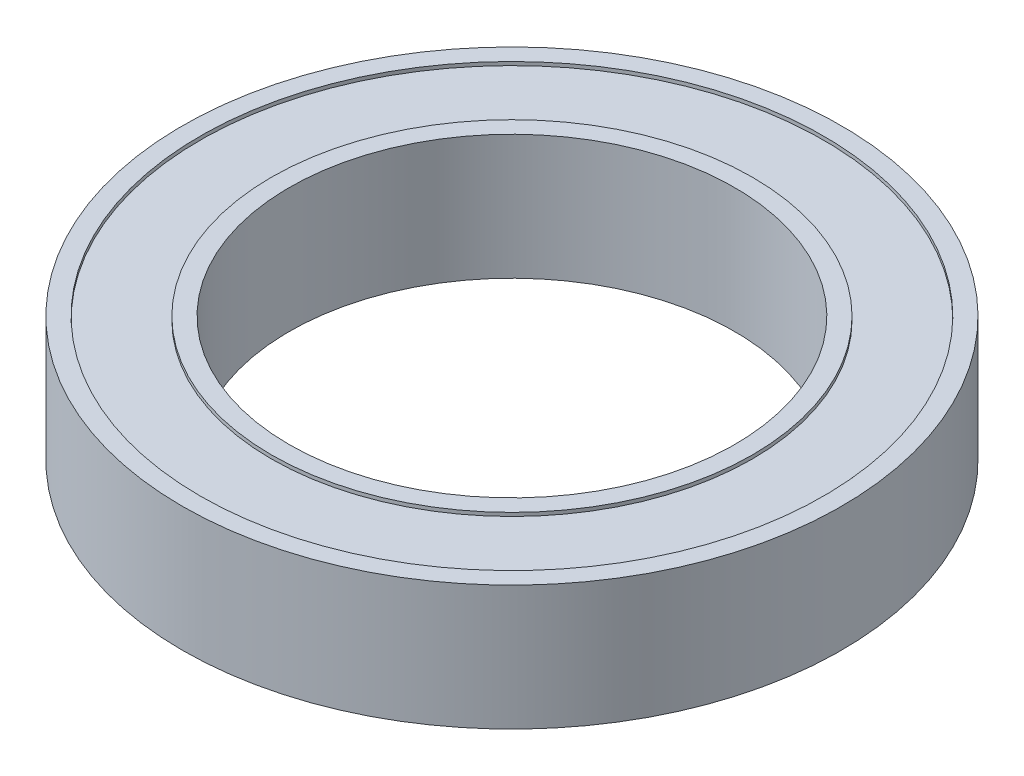
from build123d import *

# Parameters (mm, degrees)
SKETCH1_R           = 18.5
SKETCH1_R_2         = 12.5
BOSS_EXTRUDE1_DEPTH = 7
SKETCH2_R           = 17.5
SKETCH2_R_2         = 13.5
CUT_EXTRUDE1_DEPTH  = 0.2
CUT_EXTRUDE2_START  = -0.2
SKETCH3_R           = 17.5
SKETCH3_R_2         = 13.5
CUT_EXTRUDE2_DEPTH  = 0.2


with BuildPart() as part:
    # Sketch1 → Boss-Extrude1 (new body)
    with BuildSketch(Plane(origin=(0, 0, 0), x_dir=(1, 0, 0), z_dir=(0, 1, 0))):
        with Locations(Location((0, 0, 0), (0, 0, 270))):
            Circle(SKETCH1_R)
        with Locations(Location((0, 0, 0), (0, 0, 270))):
            Circle(SKETCH1_R_2, mode=Mode.SUBTRACT)
    extrude(amount=BOSS_EXTRUDE1_DEPTH)

    # Sketch2 → Cut-Extrude1 (cut)
    with BuildSketch(Plane(origin=(0, 7, 0), x_dir=(1, 0, 0), z_dir=(0, 1, 0))):
        with Locations(Location((0, 0, 0), (0, 0, 270))):
            Circle(SKETCH2_R)
        with Locations(Location((0, 0, 0), (0, 0, 270))):
            Circle(SKETCH2_R_2, mode=Mode.SUBTRACT)
    extrude(amount=-CUT_EXTRUDE1_DEPTH, mode=Mode.SUBTRACT)

    # Sketch3 → Cut-Extrude2 (cut)
    with BuildSketch(Plane.XZ.offset(CUT_EXTRUDE2_START)):
        with Locations(Location((0, 0, 0), (0, 0, 90))):
            Circle(SKETCH3_R)
        with Locations(Location((0, 0, 0), (0, 0, 90))):
            Circle(SKETCH3_R_2, mode=Mode.SUBTRACT)
    extrude(amount=CUT_EXTRUDE2_DEPTH, mode=Mode.SUBTRACT)


solid = part.part
